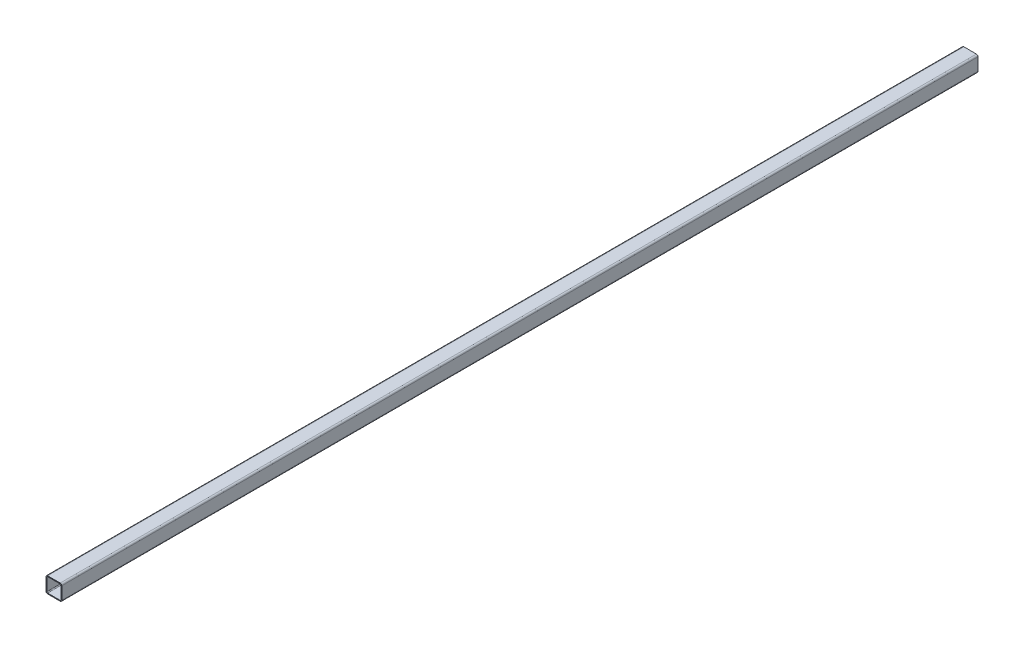
from build123d import *

# Parameters (mm, degrees)
BOSS_EXTRUDE1_DEPTH = 5800


with BuildPart() as part:
    # Sketch1 → Boss-Extrude1 (new body)
    with BuildSketch(Plane.XY):
        with BuildLine():
            Line((10, 0), (90, 0))
            ThreePointArc((90, 0), (97.071067812, 2.928932188), (100, 10))
            Line((100, 10), (100, 90))
            ThreePointArc((100, 90), (97.071067812, 97.071067812), (90, 100))
            Line((90, 100), (10, 100))
            ThreePointArc((10, 100), (2.928932188, 97.071067812), (0, 90))
            Line((0, 90), (0, 10))
            ThreePointArc((0, 10), (2.928932188, 2.928932188), (10, 0))
        make_face()
        with BuildLine():
            Line((10, 95), (90, 95))
            ThreePointArc((90, 95), (93.535533906, 93.535533906), (95, 90))
            Line((95, 90), (95, 10))
            ThreePointArc((95, 10), (93.535533906, 6.464466094), (90, 5))
            Line((90, 5), (10, 5))
            ThreePointArc((10, 5), (6.464466094, 6.464466094), (5, 10))
            Line((5, 10), (5, 90))
            ThreePointArc((5, 90), (6.464466094, 93.535533906), (10, 95))
        make_face(mode=Mode.SUBTRACT)
    extrude(amount=BOSS_EXTRUDE1_DEPTH)


solid = part.part
